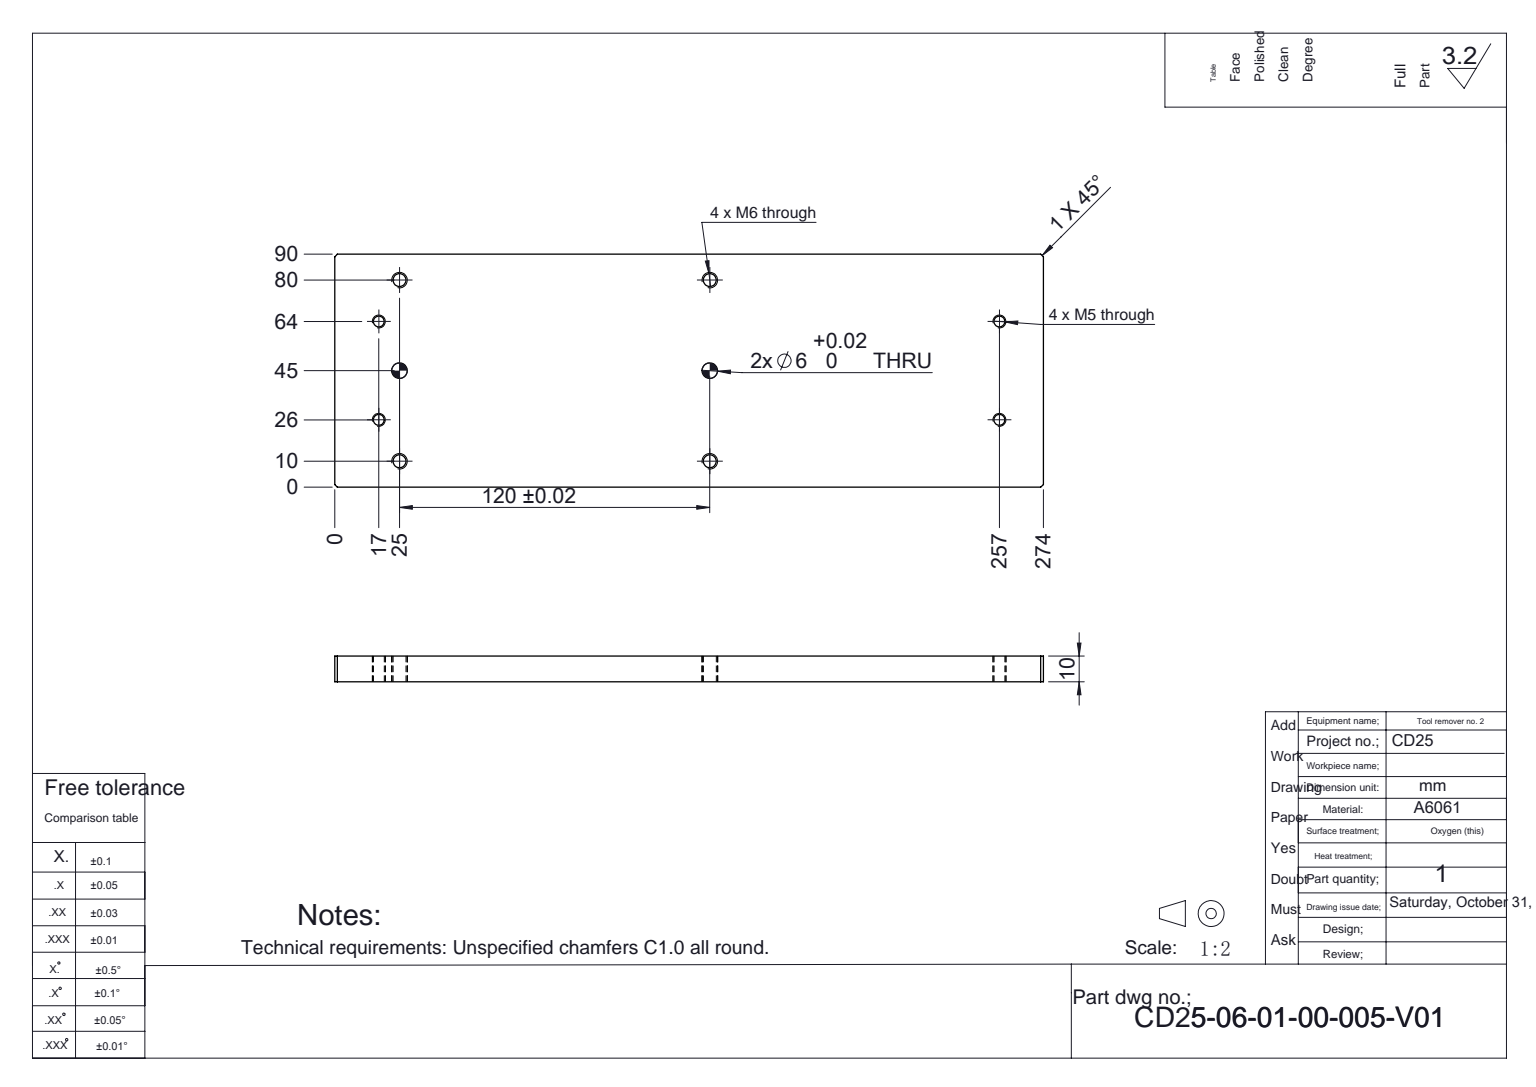
from build123d import *

# Parameters (mm, degrees)
SKETCH1_W             = 274
SKETCH1_H             = 90
BOSS_EXTRUDE1_DEPTH   = 5
M5_TAPPED_HOLE1_D     = 4.2
M6_TAPPED_HOLE1_D     = 5
F_6_0MM_BLIND_HOLE1_D = 6
CHAMFER1_SIZE         = 1


with BuildPart() as part:
    # Sketch1 → Boss-Extrude1 (new, symmetric)
    with BuildSketch(Plane.XY):
        Rectangle(SKETCH1_W, SKETCH1_H)
    extrude(amount=BOSS_EXTRUDE1_DEPTH, both=True)

    # M5 Tapped Hole1 (through all)
    with Locations(Plane.XY.offset(5)):
        with Locations((-120, 19), (-120, -19), (120, -19), (120, 19)):
            Hole(M5_TAPPED_HOLE1_D / 2)

    # M6 Tapped Hole1 (through all)
    with Locations(Plane(origin=(0, 0, -5), x_dir=(-1, 0, 0), z_dir=(0, 0, -1))):
        with Locations((112, 35), (112, -35), (-8, -35), (-8, 35)):
            Hole(M6_TAPPED_HOLE1_D / 2)

    # Ø6.0mm blind hole1 (through all)
    with Locations(Plane(origin=(0, 0, -5), x_dir=(-1, 0, 0), z_dir=(0, 0, -1))):
        with Locations((112, 0), (-8, 0)):
            Hole(F_6_0MM_BLIND_HOLE1_D / 2)

    # Chamfer1
    chamfer1_edges = [part.edges().sort_by_distance(p)[0] for p in [
        (137, -45, 0),
        (-137, -45, 0),
        (-137, 45, 0),
        (137, 45, 0),
    ]]
    chamfer(chamfer1_edges, length=CHAMFER1_SIZE)


solid = part.part
